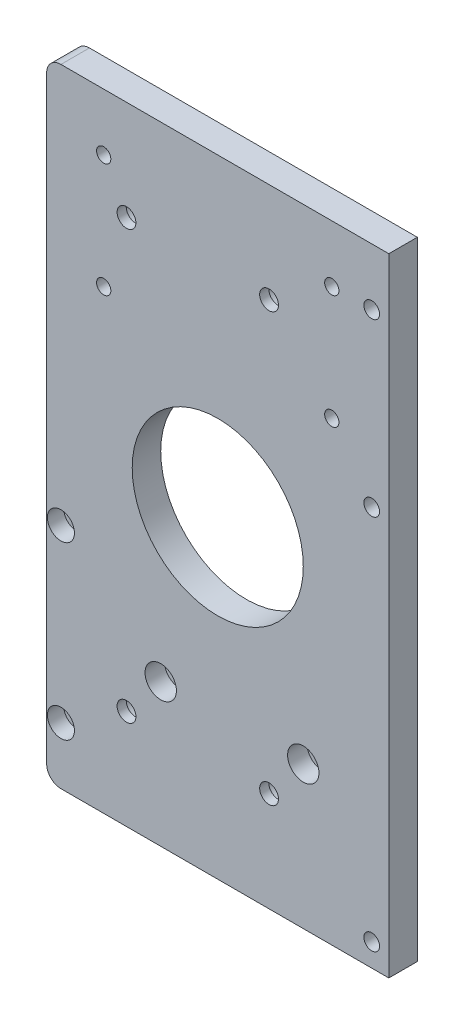
from build123d import *

# Parameters (mm, degrees)
SKETCH_1_W                = 120
SKETCH_1_H                = 220
EXTRUDE_1_DEPTH           = 10
HOLE_WIZARD_M6_1_D        = 5
HOLE_WIZARD_1_D           = 6.6
HOLE_WIZARD_1_CBORE_D     = 11
HOLE_WIZARD_1_CBORE_DEPTH = 6.8
CUT_EXTRUDE_1_REACH       = 127.698
SKETCH_6_R                = 30
HOLE_WIZARD_2_D           = 5.5
HOLE_WIZARD_2_CBORE_D     = 9.5
HOLE_WIZARD_2_CBORE_DEPTH = 5.7
HOLE_WIZARD_3_D           = 6.6
HOLE_WIZARD_3_CBORE_D     = 11
HOLE_WIZARD_3_CBORE_DEPTH = 6.8
HOLE_WIZARD_4_D           = 5.5
HOLE_WIZARD_4_CBORE_D     = 10
HOLE_WIZARD_4_CBORE_DEPTH = 5.7
FILLET_1_R                = 5


with BuildPart() as part:
    # 草图1 → 凸台-拉伸1 (new body)
    with BuildSketch(Plane.XY):
        Rectangle(SKETCH_1_W, SKETCH_1_H)
    extrude(amount=EXTRUDE_1_DEPTH)

    # M6 螺纹孔1 (through all)
    with Locations(Plane(origin=(0, 0, 0), x_dir=(-1, 0, 0), z_dir=(0, 0, -1))):
        with Locations((-40, 90), (-40, 50), (40, 90), (40, 50)):
            Hole(HOLE_WIZARD_M6_1_D / 2)

    # 打孔尺寸(%根据)内六角圆柱头螺钉的类型1 (through all)
    with Locations(Plane(origin=(0, 0, 0), x_dir=(-1, 0, 0), z_dir=(0, 0, -1))):
        with Locations((32, -75), (-18, -75), (32, 75), (-18, 75)):
            CounterBoreHole(HOLE_WIZARD_1_D / 2, HOLE_WIZARD_1_CBORE_D / 2, HOLE_WIZARD_1_CBORE_DEPTH)

    # 草图6 → 切除-拉伸1 (cut, up to next)
    with BuildSketch(Plane(origin=(0, 0, 0), x_dir=(-1, 0, 0), z_dir=(0, 0, -1)), mode=Mode.PRIVATE) as cut_extrude_1_sk1:
        Circle(SKETCH_6_R)
    cut_extrude_1_tool1 = extrude(cut_extrude_1_sk1.sketch, amount=-CUT_EXTRUDE_1_REACH, mode=Mode.PRIVATE) & part.part
    add(cut_extrude_1_tool1.solids().sort_by_distance((0, 0, 0))[0], mode=Mode.SUBTRACT)

    # 打孔尺寸(%根据)内六角圆柱头螺钉的类型2 (through all)
    with Locations(Plane.XY.offset(10)):
        with Locations((-55, -30), (-55, -90)):
            CounterBoreHole(HOLE_WIZARD_2_D / 2, HOLE_WIZARD_2_CBORE_D / 2, HOLE_WIZARD_2_CBORE_DEPTH)

    # 打孔尺寸(%根据)内六角圆柱头螺钉的类型3 (through all)
    with Locations(Plane.XY.offset(10)):
        with Locations((-20, -60), (30, -60)):
            CounterBoreHole(HOLE_WIZARD_3_D / 2, HOLE_WIZARD_3_CBORE_D / 2, HOLE_WIZARD_3_CBORE_DEPTH)

    # 打孔尺寸(%根据)内六角圆柱头螺钉的类型4 (through all)
    with Locations(Plane(origin=(0, 0, 0), x_dir=(-1, 0, 0), z_dir=(0, 0, -1))):
        with Locations((-54, 30), (-54, 90), (-54, -102)):
            CounterBoreHole(HOLE_WIZARD_4_D / 2, HOLE_WIZARD_4_CBORE_D / 2, HOLE_WIZARD_4_CBORE_DEPTH)

    # 圆角1
    fillet_1_edges = [part.edges().sort_by_distance(p)[0] for p in [
        (-60, 110, 5),
        (-60, -110, 5),
    ]]
    fillet(fillet_1_edges, radius=FILLET_1_R)


solid = part.part
